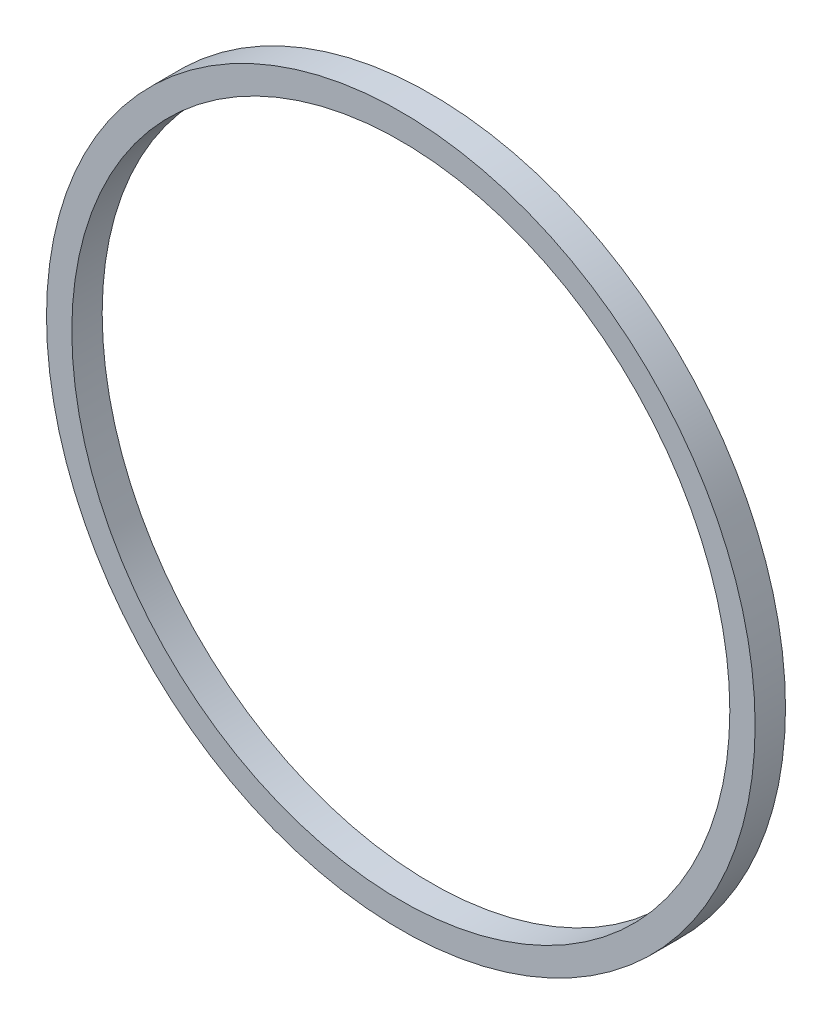
SolidWorks part; units mm, degrees
ref_plane "前视基准面" through (0, 0, 0) normal (0, 0, 1) x (1, 0, 0)
ref_plane "上视基准面" through (0, 0, 0) normal (0, 1, 0) x (1, 0, 0)
ref_plane "右视基准面" through (0, 0, 0) normal (1, 0, 0) x (0, 0, -1)
sketch "草图1" plane through (0, 0, 0) normal (0, 0, 1) x (1, 0, 0)
  circle A0 centre (0, 0) radius 32.5
  circle A1 centre (0, 0) radius 35
  dimension "D1" = 65
  dimension "D2" = 70
extrude "凸台-拉伸1" add sketch "草图1" along normal blind 3
